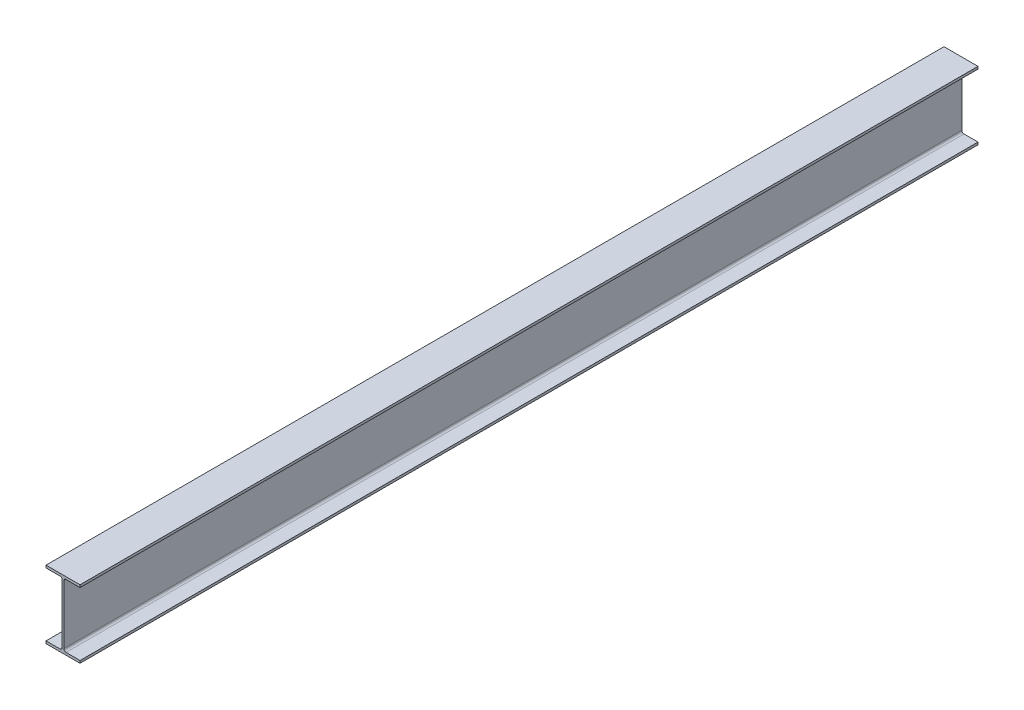
from build123d import *

# Parameters (mm, degrees)
BOSS_EXTRUDE1_DEPTH = 3300


with BuildPart() as part:
    # Sketch1 → Boss-Extrude1 (new body)
    with BuildSketch(Plane.XY):
        with BuildLine():
            Line((62.5, 0), (-62.5, 0))
            Line((-62.5, 0), (-62.5, 9))
            Line((-62.5, 9), (-11, 9))
            ThreePointArc((-11, 9), (-5.343145751, 11.343145751), (-3, 17))
            Line((-3, 17), (-3, 233))
            ThreePointArc((-3, 233), (-5.343145751, 238.656854249), (-11, 241))
            Line((-11, 241), (-62.5, 241))
            Line((-62.5, 241), (-62.5, 250))
            Line((-62.5, 250), (62.5, 250))
            Line((62.5, 250), (62.5, 241))
            Line((62.5, 241), (11, 241))
            ThreePointArc((11, 241), (5.343145751, 238.656854249), (3, 233))
            Line((3, 233), (3, 17))
            ThreePointArc((3, 17), (5.343145751, 11.343145751), (11, 9))
            Line((11, 9), (62.5, 9))
            Line((62.5, 9), (62.5, 0))
        make_face()
    extrude(amount=BOSS_EXTRUDE1_DEPTH)


solid = part.part
